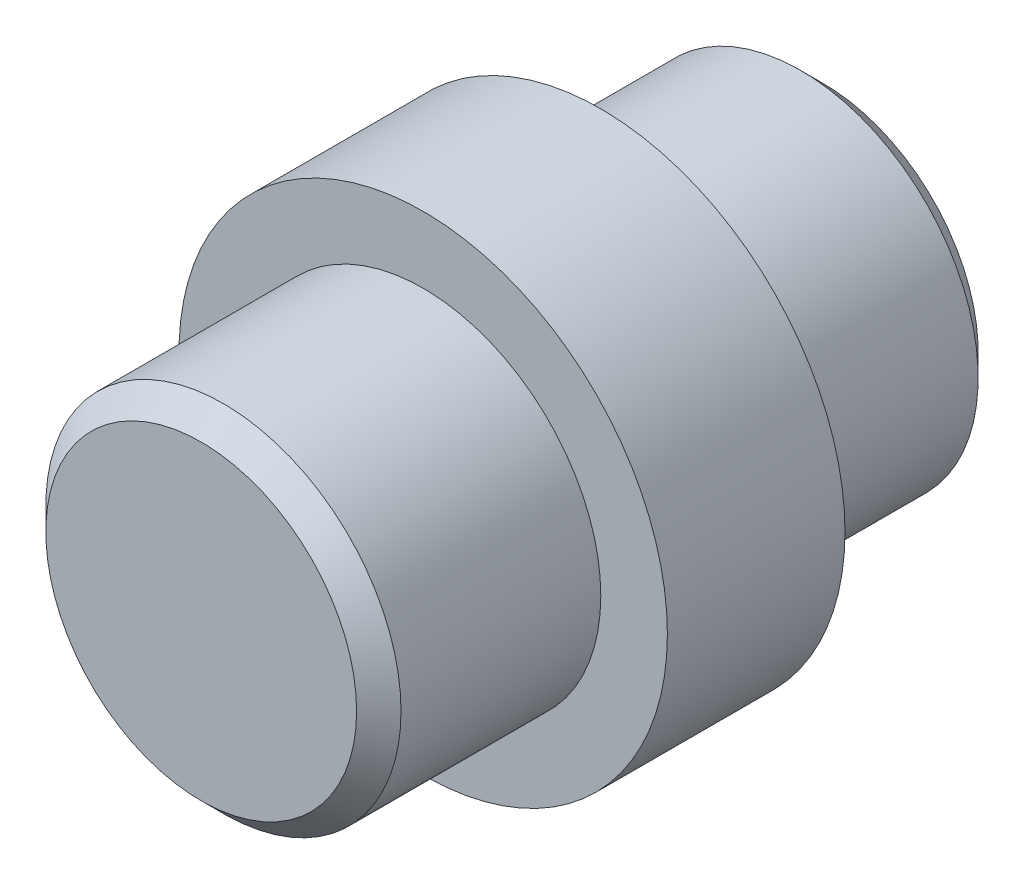
SolidWorks part; units mm, degrees
ref_plane "Front Plane" through (0, 0, 0) normal (0, 0, 1) x (1, 0, 0)
ref_plane "Top Plane" through (0, 0, 0) normal (0, 1, 0) x (1, 0, 0)
ref_plane "Right Plane" through (0, 0, 0) normal (1, 0, 0) x (0, 0, -1)
other "Configuration Table"
sketch "Sketch1" plane through (0, 0, 0) normal (0, 0, 1) x (1, 0, 0)
  circle A0 centre (0, 0) radius 11
  dimension "D1" = 22
extrude "Boss-Extrude1" add sketch "Sketch1" along normal blind 8
sketch "Sketch2" plane through (0, 0, 8) normal (0, 0, 1) x (1, 0, 0)
  circle A0 centre (0, 0) radius 8
  dimension "D1" = 16
extrude "Boss-Extrude2" add sketch "Sketch2" along normal blind 10
sketch "Sketch3" plane through (0, 0, 0) normal (0, 0, -1) x (-1, 0, 0)
  circle A0 centre (0, 0) radius 8
  dimension "D1" = 16
extrude "Boss-Extrude3" add sketch "Sketch3" along normal blind 10
chamfer "Chamfer1" distance 1 angle 45 2 edges at (8, 0, 18) (-8, 0, -10)
